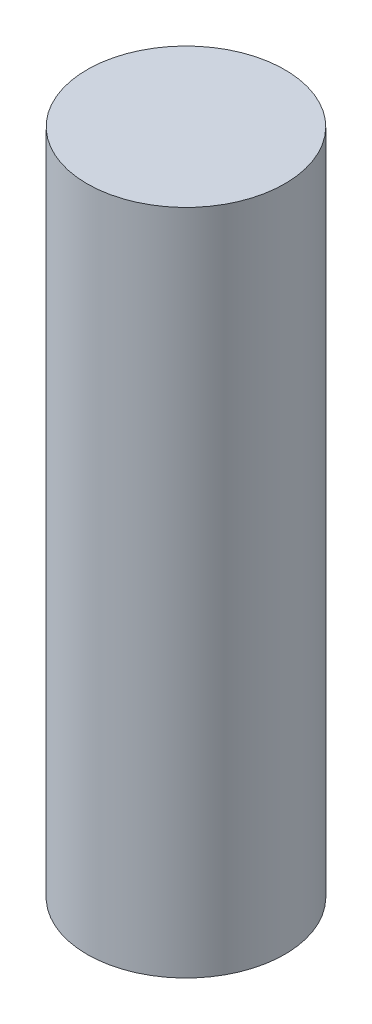
SolidWorks part; units mm, degrees
ref_plane "Front Plane" through (0, 0, 0) normal (0, 0, 1) x (1, 0, 0)
ref_plane "Top Plane" through (0, 0, 0) normal (0, 1, 0) x (1, 0, 0)
ref_plane "Right Plane" through (0, 0, 0) normal (1, 0, 0) x (0, 0, -1)
sketch "Sketch1" plane through (0, 0, 0) normal (0, 1, 0) x (1, 0, 0)
  circle A0 centre (0, 0) radius 8
  dimension "D1" = 16
extrude "Boss-Extrude1" add sketch "Sketch1" along normal blind 54
